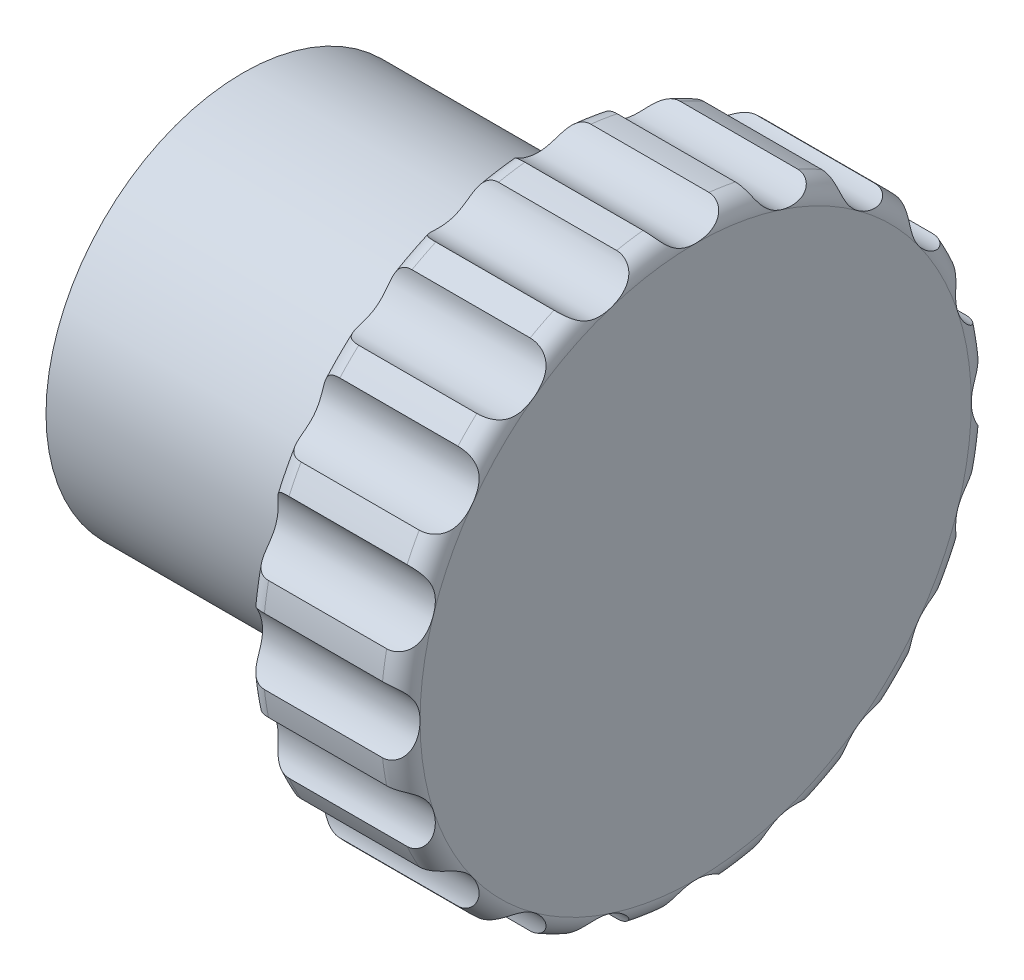
from build123d import *

# Parameters (mm, degrees)
SKETCH_2_R          = 2
CUT_EXTRUDE_1_DEPTH = 8


with BuildPart() as part:
    # Sketch 1 → Revolve 1 (revolve)
    with BuildSketch(Plane.XY, mode=Mode.PRIVATE) as revolve_1_sk:
        with BuildLine():
            Line((0, 0), (0, 10))
            Line((0, 10), (15, 10))
            Line((15, 10), (15, 14))
            ThreePointArc((15, 14), (15.292893219, 14.707106781), (16, 15))
            Line((16, 15), (22, 15))
            ThreePointArc((22, 15), (22.707106781, 14.707106781), (23, 14))
            Line((23, 14), (23, 0))
            Line((23, 0), (0, 0))
        make_face()
    revolve(revolve_1_sk.sketch.rotate(Axis((-9.102564103, 0, 0), (1, 0, 0)), 90), axis=Axis((-9.102564103, 0, 0), (1, 0, 0)))

    # Sketch 2 → Cut-Extrude 1 (cut)
    with BuildSketch(Plane(origin=(23, 0, 0), x_dir=(0, 0, -1), z_dir=(1, 0, 0))):
        with Locations((0, 16)):
            Circle(SKETCH_2_R)
        with Locations((4.94427191, 15.216904261)):
            Circle(SKETCH_2_R)
        with Locations((9.404564037, 12.94427191)):
            Circle(SKETCH_2_R)
        with Locations((12.94427191, 9.404564037)):
            Circle(SKETCH_2_R)
        with Locations((15.216904261, 4.94427191)):
            Circle(SKETCH_2_R)
        with Locations((16, 0)):
            Circle(SKETCH_2_R)
        with Locations((15.216904261, -4.94427191)):
            Circle(SKETCH_2_R)
        with Locations((12.94427191, -9.404564037)):
            Circle(SKETCH_2_R)
        with Locations((9.404564037, -12.94427191)):
            Circle(SKETCH_2_R)
        with Locations((4.94427191, -15.216904261)):
            Circle(SKETCH_2_R)
        with Locations((0, -16)):
            Circle(SKETCH_2_R)
        with Locations((-4.94427191, -15.216904261)):
            Circle(SKETCH_2_R)
        with Locations((-9.404564037, -12.94427191)):
            Circle(SKETCH_2_R)
        with Locations((-12.94427191, -9.404564037)):
            Circle(SKETCH_2_R)
        with Locations((-15.216904261, -4.94427191)):
            Circle(SKETCH_2_R)
        with Locations((-16, 0)):
            Circle(SKETCH_2_R)
        with Locations((-15.216904261, 4.94427191)):
            Circle(SKETCH_2_R)
        with Locations((-12.94427191, 9.404564037)):
            Circle(SKETCH_2_R)
        with Locations((-9.404564037, 12.94427191)):
            Circle(SKETCH_2_R)
        with Locations((-4.94427191, 15.216904261)):
            Circle(SKETCH_2_R)
    extrude(amount=-CUT_EXTRUDE_1_DEPTH, mode=Mode.SUBTRACT)


solid = part.part
